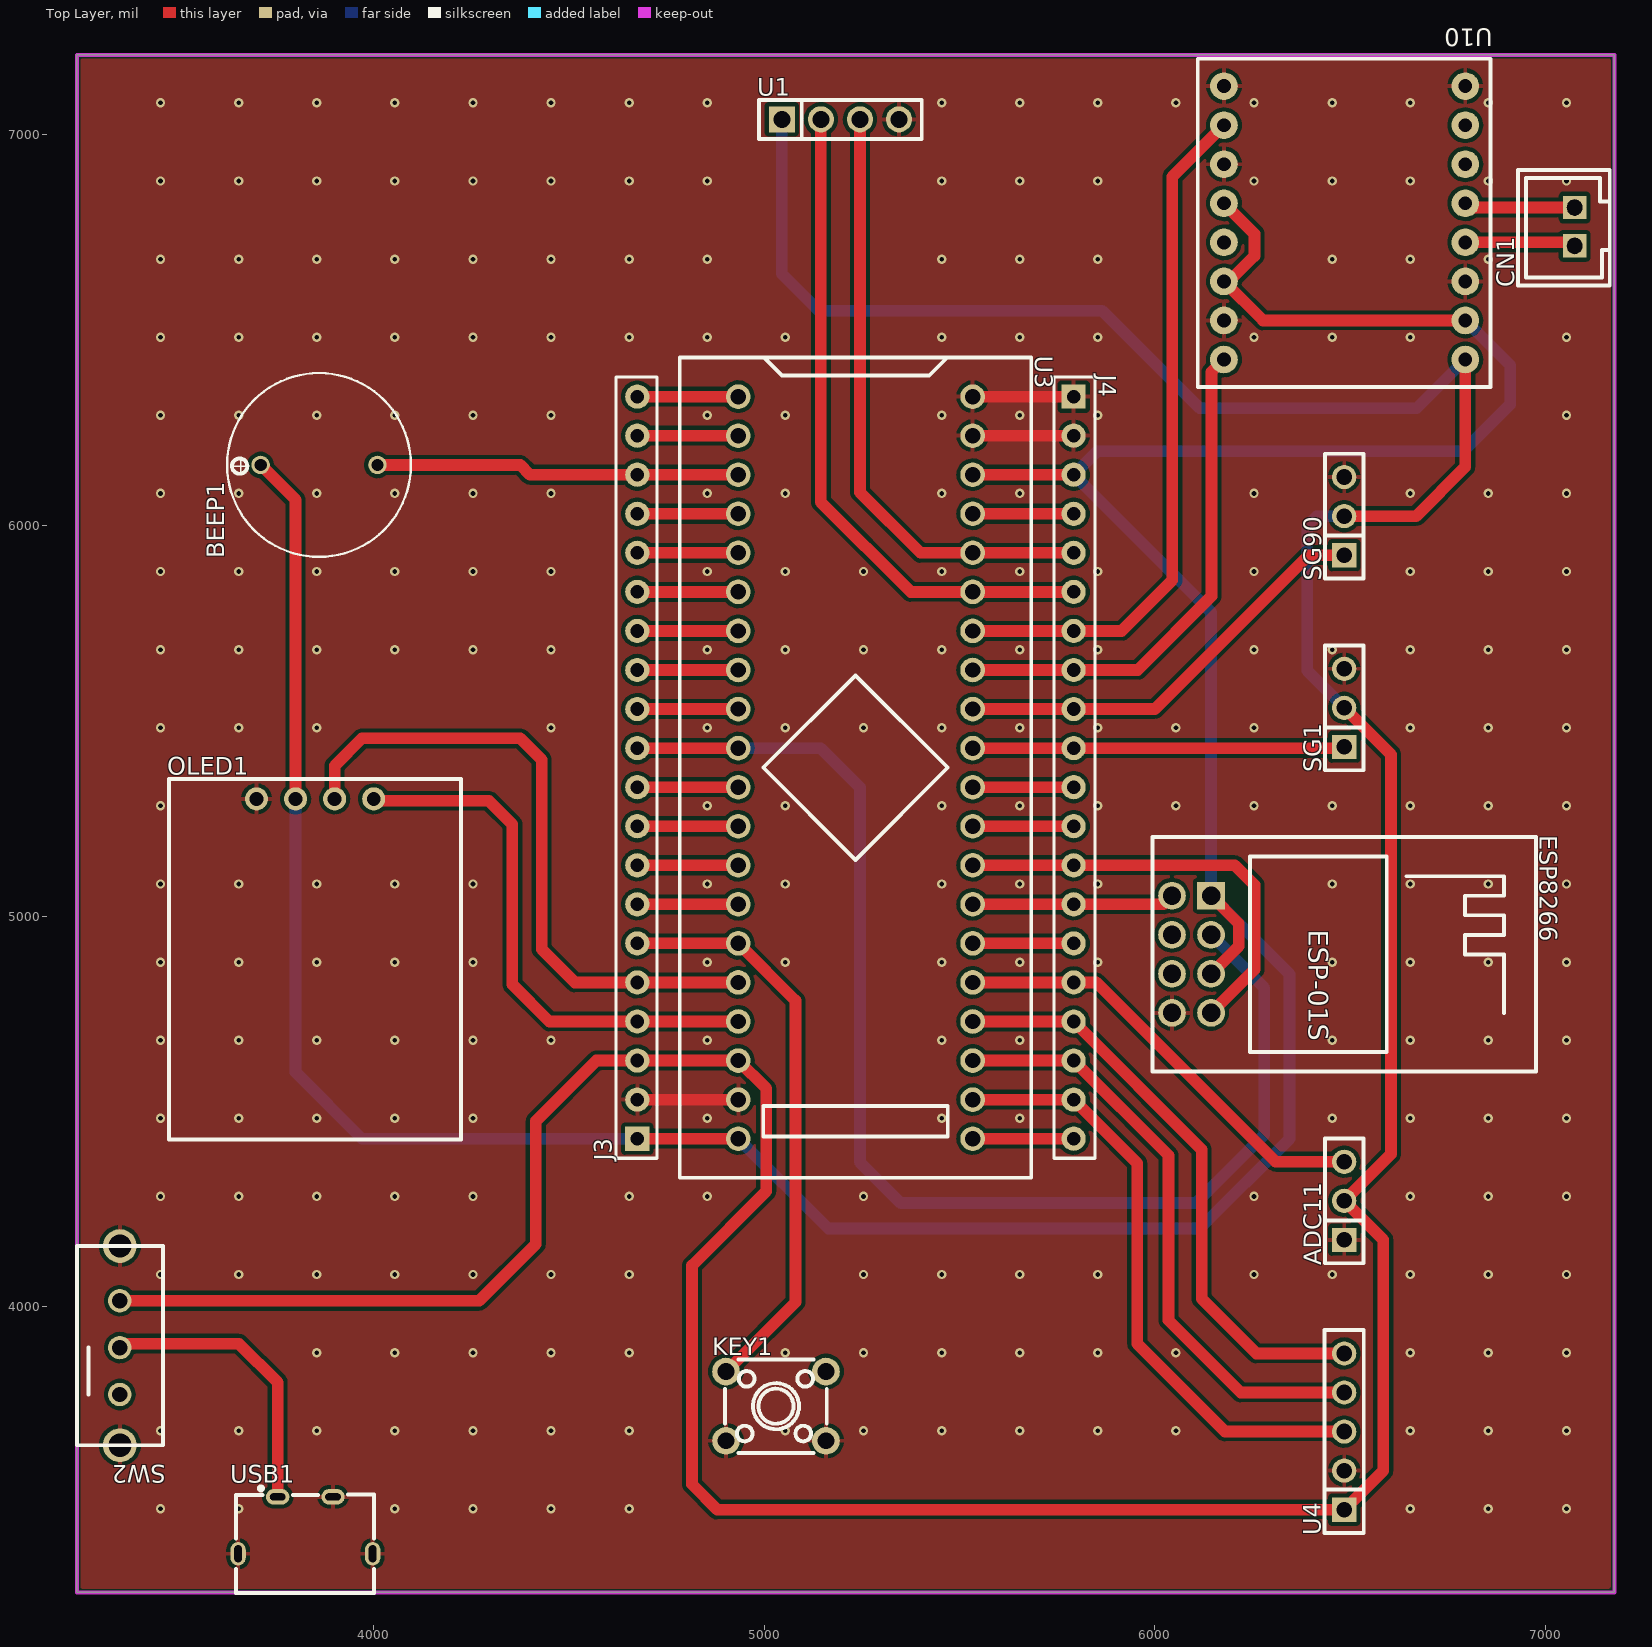
[diagram p0: Top Layer view]
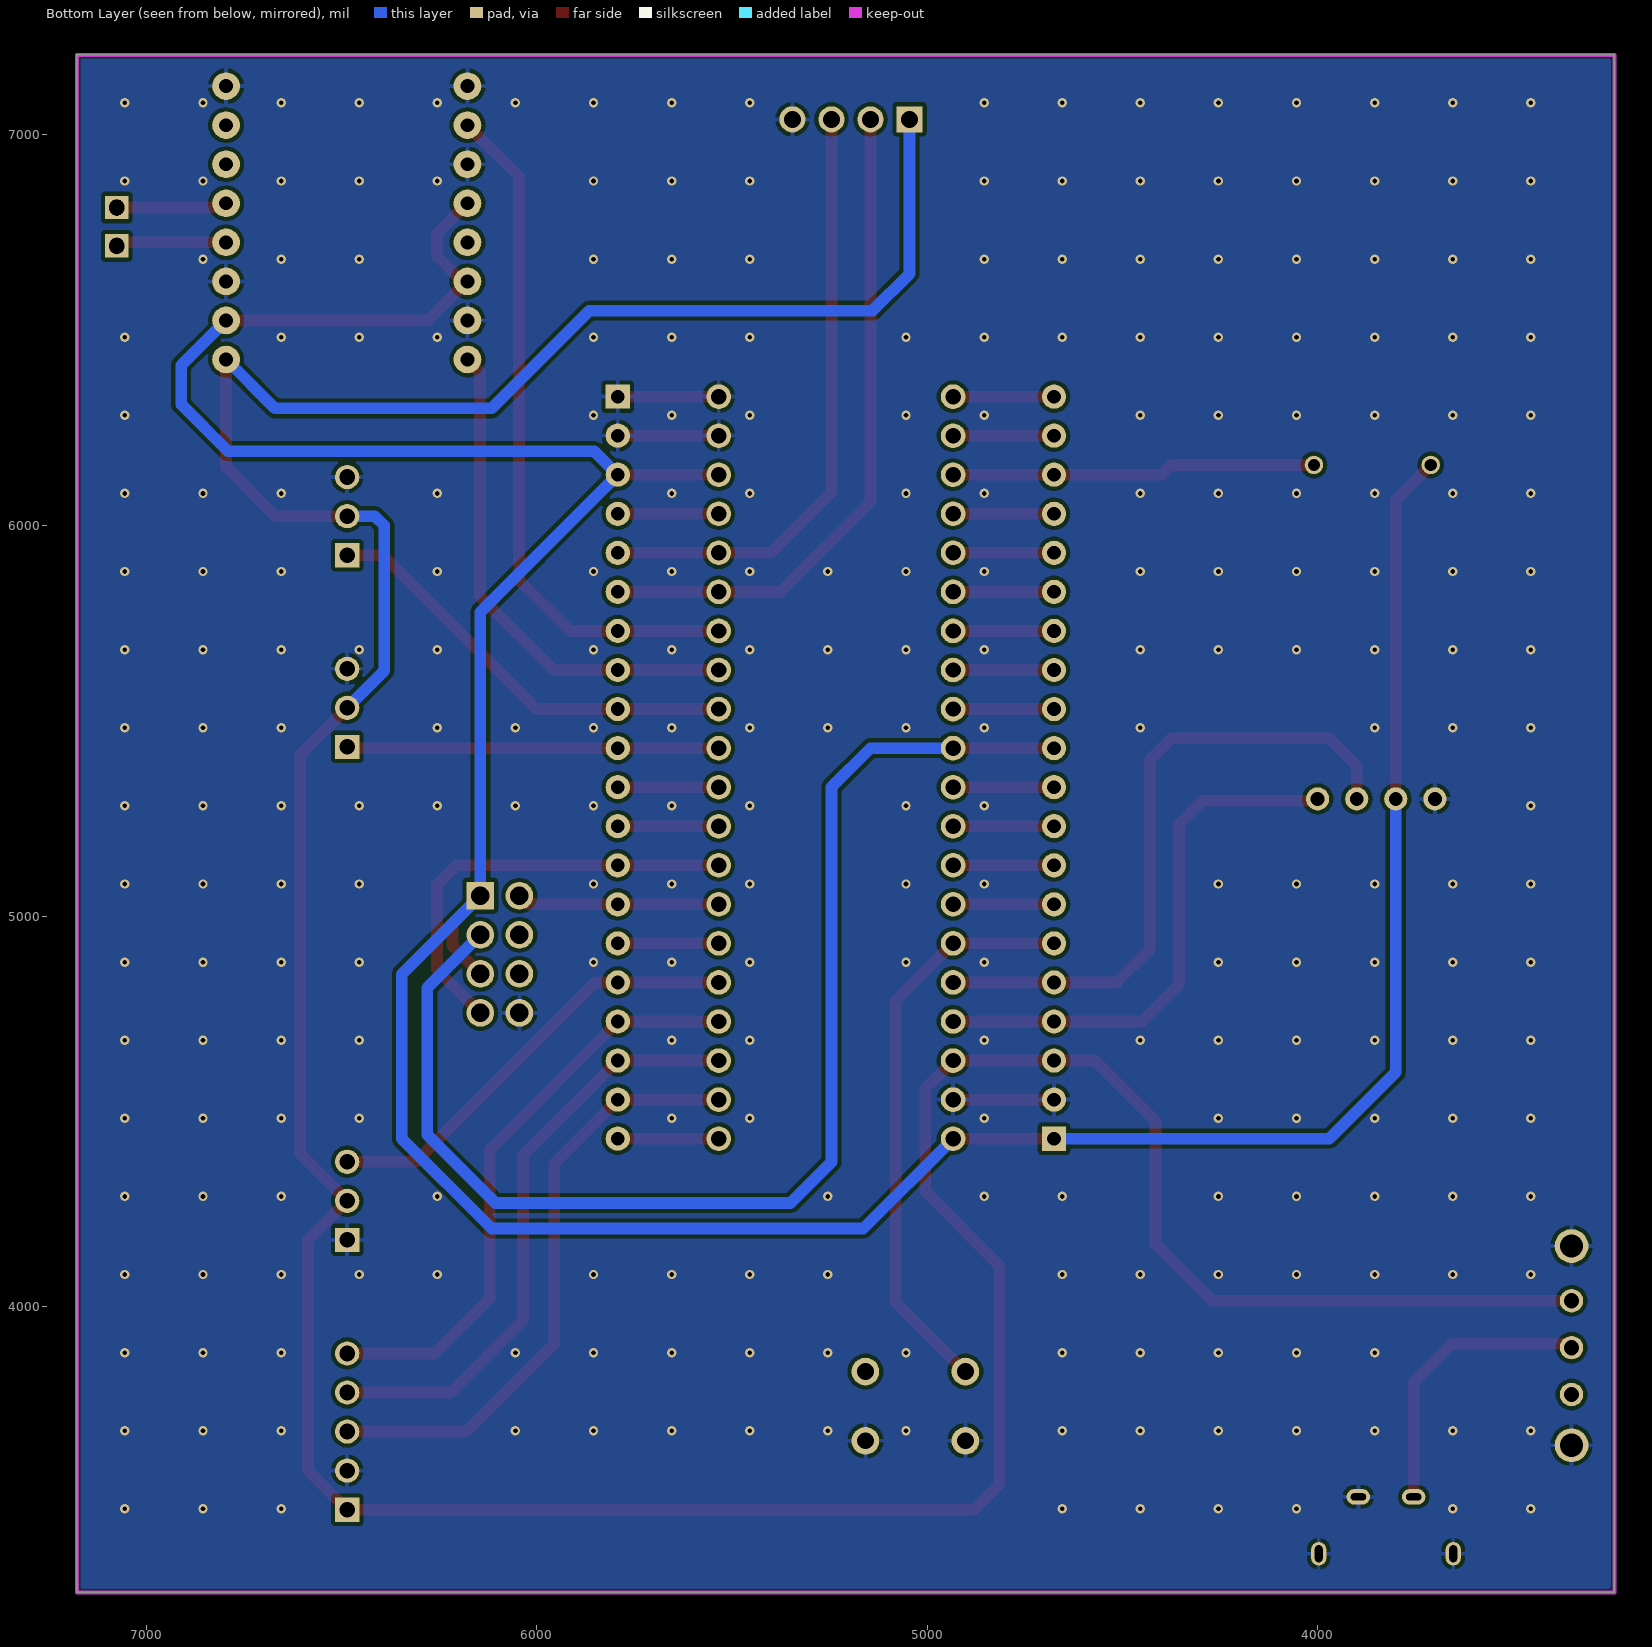
[diagram p1: Bottom Layer view, seen from below]
# Altium PCB MISC49936.pcbdoc
Units mil, origin at the board's own origin, x right, y up, seen from the top; angles counter-clockwise.
Board outline 3937.01 x 3937.01 mil, 2 copper layers (Top Layer, Bottom Layer), stack 62.206 mil thick; 16 components, 42 nets, 143 pads, 269 vias.

## Layer stack, top to bottom
Top Solder Mask Layer: solder mask 0.394, Dk 3.3
Top Layer: signal copper 1.379
Dielectric1: surface 59.449, FR4, Dk 4.5
Bottom Layer: signal copper 1.378
Bottom Solder Mask Layer: solder mask 0.394, Dk 3.3

## Board outline
3240,7205 3240,3267.99 7177.01,3267.99 7177.01,7205

## Design rules (kind name [scope] priority, off if disabled: settings)
BoardOutlineClearance copperThickness2oz_1 [All] p2 off: genericclearance=7.99 ignorepadtopadclearanceinfootprint=FALSE except(0: Arc-SplitContinuation Track-SplitContinuation SMDPad-SplitContinuation THPad-SplitContinuation Via-SplitContinuation Fill-SplitContinuation Region-SplitContinuation Poly-SplitContinuation Text-SplitContinuation Hole-SplitContinuation; 5.98: Arc-CutoutEdge SMDPad-CutoutEdge THPad-CutoutEdge Via-CutoutEdge Fill-CutoutEdge Region-CutoutEdge Text-CutoutEdge; 6.93: Hole-OutlineEdge Hole-CutoutEdge; 10: Poly-OutlineEdge Poly-CutoutEdge; 11.81: Arc-OutlineEdge Track-OutlineEdge SMDPad-OutlineEdge THPad-OutlineEdge Via-OutlineEdge Fill-OutlineEdge Region-OutlineEdge Text-OutlineEdge Track-CutoutEdge)
BoardOutlineClearance copperThickness1oz_1 [All] p4: genericclearance=4.02 ignorepadtopadclearanceinfootprint=FALSE except(0: Arc-SplitContinuation Track-SplitContinuation SMDPad-SplitContinuation THPad-SplitContinuation Via-SplitContinuation Fill-SplitContinuation Region-SplitContinuation Poly-SplitContinuation Text-SplitContinuation Hole-SplitContinuation; 6: SMDPad-CutoutEdge THPad-CutoutEdge Via-CutoutEdge Fill-CutoutEdge Region-CutoutEdge Text-CutoutEdge; 6.93: Hole-OutlineEdge Hole-CutoutEdge; 10: Poly-OutlineEdge Poly-CutoutEdge; 11.8: Arc-OutlineEdge Track-OutlineEdge SMDPad-OutlineEdge THPad-OutlineEdge Via-OutlineEdge Fill-OutlineEdge Region-OutlineEdge Text-OutlineEdge; 11.81: Arc-CutoutEdge Track-CutoutEdge)
Clearance copperThickness2oz [All] p1 off: gap=7.99 ignorepadtopadclearanceinfootprint=FALSE except(5.98: SMDPad-Track SMDPad-SMDPad THPad-Track SMDPad-THPad THPad-THPad Track-Via SMDPad-Via THPad-Via Via-Via Fill-Track Region-Track Fill-SMDPad Region-SMDPad Fill-THPad Region-THPad Fill-Via Region-Via Fill-Fill Fill-Region Region-Region Arc-Track Arc-SMDPad Arc-THPad Arc-Via Fill-Arc Region-Arc Arc-Arc Text-Track SMDPad-Text Text-THPad Text-Via Fill-Text Region-Text Arc-Text Text-Text; 6.93: Hole-Track Hole-SMDPad Hole-THPad Hole-Via Fill-Hole Region-Hole Hole-Arc Hole-Text; 10: Poly-Track Poly-SMDPad Poly-THPad Poly-Via Poly-Fill Poly-Region Poly-Poly Poly-Arc Poly-Text Poly-Hole)
Clearance copperThickness1oz [All] p3: gap=4.02 ignorepadtopadclearanceinfootprint=FALSE except(5.98: SMDPad-Track SMDPad-SMDPad THPad-Track SMDPad-THPad THPad-THPad Track-Via SMDPad-Via THPad-Via Via-Via Fill-Track Region-Track Fill-SMDPad Region-SMDPad Fill-THPad Region-THPad Fill-Via Region-Via Fill-Fill Fill-Region Region-Region; 6: Arc-Track Arc-SMDPad Arc-THPad Arc-Via Fill-Arc Region-Arc Arc-Arc Text-Track SMDPad-Text Text-THPad Text-Via Fill-Text Region-Text Arc-Text Text-Text; 6.93: Hole-Track Hole-SMDPad Hole-THPad Hole-Via Fill-Hole Region-Hole Hole-Arc Hole-Text; 10: Poly-Track Poly-SMDPad Poly-THPad Poly-Via Poly-Fill Poly-Region Poly-Poly Poly-Arc Poly-Text Poly-Hole)
DiffPairsRouting differentialPair [All] p1: maxlimit=6 minlimit=6 mostfreqgap=6 toplayer_minwidth=5 toplayer_prefwidth=10 toplayer_maxwidth=100 toplayer_mingap=6 toplayer_prefgap=6 toplayer_maxgap=6 bottomlayer_minwidth=5 bottomlayer_prefwidth=10 bottomlayer_maxwidth=100 bottomlayer_mingap=6 bottomlayer_prefgap=6 bottomlayer_maxgap=6 maxuncoupledlength=10
HoleToHoleClearance otherClearance [All] p1: gap=11.81 allowstackedmicrovias=TRUE
Length netLength [All] p1: minlimit=0 maxlimit=0
MatchedLengths netLengthTolerance [All] p1: tolerance=1000
PasteMaskExpansion pasteMaskExpansion [All] p1: expansion=0
PlaneConnect innerPlane [All] p1: planeconnectstyle=Relief reliefexpansion=20 reliefentries=4 reliefconductorwidth=10 reliefairgap=10
PolygonConnect copperRegion [(InNet('GND'))] p1: connectstyle=Relief reliefconductorwidth=10 reliefentries=4 polygonreliefangle="90 Angle" airgapwidth=10 via.connectstyle=Relief via.reliefconductorwidth=10 via.reliefentries=4 via.polygonreliefangle="90 Angle" via.airgapwidth=10
RoutingVias viaSize [All] p1: holewidth=12.01 width=24.02 viastyle="Through Hole" minholewidth=11.81 minwidth=19.68 maxholewidth=248.03 maxwidth=393.7
SolderMaskExpansion solderMaskExpansion [IsVia] p1: expansion=-1000 istentingtop=TRUE
SolderMaskExpansion solderMaskExpansion [All] p2: expansion=2 istentingtop=FALSE
Width copperThickness2oz_2 [All] p1 off: maxlimit=100 minlimit=8 preferedwidth=10
Width copperThickness1oz_2 [All] p2: maxlimit=100 minlimit=5 preferedwidth=10

## Components (designator, comment, footprint, x,y, rotation, side; value= is the part's Value field where it differs from the comment)
ADC11 "MQ135" HDR-TH_3P-P2.54-V-F 6485,4270.87 r90 top
BEEP1 "Buzzer" BUZ-TH_BD11.8-P7.60_XHXDZ-TMB12065 3860,6155 r90 top
CN1 "XH2.54-2PIN-straight pin" CONN-TH_XH2.54-2P 7075,6765 r90 top
ESP8266 "ESP-01S module" WIFIM-TH_ESP-01S 6094,4901.99 r270 top
J3 "HDR-M-2.54_1x20" HDR-M-2.54_1X20 4675,5380 r90 top
J4 "HDR-M-2.54_1x20" HDR-M-2.54_1X20 5792.09,5380 r270 top
KEY1 "K4-6×6_TH" KEY-TH_4P-L6.0-W6.0-P4.50-LS6.5 5030,3745 r0 top
OLED1 "0.96 OLED IIC COPY" OLED-TH_4P-L23.44-W19.0_ER-OLEDM0.66-1W-I2C 3850,5300 r0 top
SG1 "Servo" HDR-TH_3P-P2.54-V-F 6485,5533.11 r90 top
SG90 "Servo" HDR-TH_3P-P2.54-V-F 6485,6023.98 r90 top
SW2 "SK-12E12-G5" SW-TH_SK-12E12-G5 3350,3900 r180 top
U1 "HX711" HDR-TH_4P-P2.54-V-F 5195,7040 r0 top
U3 "STM32F103C8T6-Card" CONN-TH_L53.3-W22.9_STM32F103C8T6-CARD 5233.54,5380 r270 top
U4 "Clock DS1302" HDR-TH_5P-P2.54-V-F 6485,3680 r90 top
U10 "TB6612FNG" tb6612 6795,6425 r180 top
USB1 "KH-TYPE-C-2P" USB-SMD_KH-TYPE-C-2P 3825,3440 r0 top

## Footprints (in the part's own frame and the unit in brackets; to place one, negate y for a bottom-side part, rotate by r counter-clockwise, add the part's x,y. Pads: shape width x height; smd on the part's side, far side on the other; paste and mask are expansions set on the pad)
BUZ-TH_BD11.8-P7.60_XHXDZ-TMB12065 [mm]
  round 1.201 hole 0.801: 1(0,3.8) 2(0,-3.8)
  silkscreen extent -5.98,-5.98 5.98,5.98
CONN-TH_L53.3-W22.9_STM32F103C8T6-CARD [mm]
  round 1.6 hole 1: 1(-24.13,-7.62) 2(-21.59,-7.62) 3(-19.05,-7.62) 4(-16.51,-7.62) 5(-13.97,-7.62) 6(-11.43,-7.62) 7(-8.89,-7.62) 8(-6.35,-7.62) 9(-3.81,-7.62) 10(-1.27,-7.62) 11(1.27,-7.62) 12(3.81,-7.62) 13(6.35,-7.62) 14(8.89,-7.62) 15(11.43,-7.62) 16(13.97,-7.62) 17(16.51,-7.62) 18(19.05,-7.62) 19(21.59,-7.62) 20(24.13,-7.62) 21(24.13,7.62) 22(21.59,7.62) 23(19.05,7.62) 24(16.51,7.62) 25(13.97,7.62) 26(11.43,7.62) 27(8.89,7.62) 28(6.35,7.62) 29(3.81,7.62) 30(1.27,7.62) 31(-1.27,7.62) 32(-3.81,7.62) 33(-6.35,7.62) 34(-8.89,7.62) 35(-11.43,7.62) 36(-13.97,7.62) 37(-16.51,7.62) 38(-19.05,7.62) 39(-21.59,7.62) 40(-24.13,7.62)
  silkscreen extent -26.67,-11.43 26.67,11.43
CONN-TH_XH2.54-2P [mil]
  rect 60x60 hole 39.37 slot 41.34 at 0 deg paste+0 mask+1.97: 1(-49.22,0) 2(49.21,0)
  silkscreen extent -150,-90 145,145
HDR-M-2.54_1X20 [mil]
  rect 62x62 hole 35: 1(-950,0)
  round 62 hole 35: 2(-850,0) 3(-750,0) 4(-650,0) 5(-550,0) 6(-450,0) 7(-350,0) 8(-250,0) 9(-150,0) 10(-50,0) 11(50,0) 12(150,0) 13(250,0) 14(350,0) 15(450,0) 16(550,0) 17(650,0) 18(750,0) 19(850,0) 20(950,0)
  silkscreen extent -1000,-50 1000,55
HDR-TH_3P-P2.54-V-F [mil]
  rect 62x62 hole 40.16: 1(-100,0)
  round 62 hole 40.16: 2(0,0) 3(100,0)
  silkscreen extent -160,-49 160,49
HDR-TH_4P-P2.54-V-F [mm]
  rect 1.7x1.7 hole 1.1: 1(-3.81,0)
  round 1.7 hole 1.1: 2(-1.27,0) 3(1.27,0) 4(3.81,0)
  silkscreen extent -5.29,-1.27 5.29,1.27
HDR-TH_5P-P2.54-V-F [mil]
  rect 62x62 hole 40.16: 1(-200,0)
  round 62 hole 40.16: 2(-100,0) 3(0,0) 4(100,0) 5(200,0)
  silkscreen extent -260,-50 260,50
KEY-TH_4P-L6.0-W6.0-P4.50-LS6.5 [mm]
  round 1.8 hole 1.1: 1(-3.251,-2.25) 2(3.251,-2.25) 3(3.251,2.25) 4(-3.251,2.25)
  silkscreen extent -3.3,-3.05 3.3,3.05
OLED-TH_4P-L23.44-W19.0_ER-OLEDM0.66-1W-I2C [mm]
  round 1.5 hole 0.9 paste+0 mask+0.05: 1(-3.81,0) 2(-1.27,0) 3(1.27,0) 4(3.81,0)
  silkscreen extent -9.5,-22.15 9.5,1.3
SW-TH_SK-12E12-G5 [mil]
  round 60 hole 39.37: 1(0,125) 2(0,5) 3(0,-115)
  round 86.61 hole 59.06: 4(0,-255) 5(0,255)
  silkscreen extent -110,-255 110,255
tb6612 [mm]
  round 1.8 hole 0.9: 1(0,0) 2(0,-2.54) 3(0,-5.08) 4(0,-7.62) 5(0,-10.16) 6(0,-12.7) 7(0,-15.24) 8(0,-17.78) 9(15.697,-17.78) 10(15.697,-15.24) 11(15.697,-12.7) 12(15.697,-10.16) 13(15.697,-7.62) 14(15.697,-5.08) 15(15.697,-2.54) 16(15.697,0)
  silkscreen extent -1.65,-19.56 17.4,1.78
USB-SMD_KH-TYPE-C-2P [mm]
  oval 1.524x1 hole 0.45 slot 1 at 0 deg paste+0 mask+0.05: 1(-1.8,1.85) 2(1.8,1.85)
  oval 1x1.524 hole 0.5 slot 1.1 at 90 deg paste+0 mask+0.05: 3(4.375,-1.85) 4(-4.375,-1.85)
  silkscreen extent -4.5,-4.41 4.46,2.53
WIFIM-TH_ESP-01S [mm]
  rect 1.8x1.8 hole 1.2: 1(-3.81,1.27)
  round 1.8 hole 1.2: 2(-1.27,1.27) 3(1.27,1.27) 4(3.81,1.27) 5(3.81,-1.27) 6(1.27,-1.27) 7(-1.27,-1.27) 8(-3.81,-1.27)
  silkscreen extent -7.62,-2.54 7.62,22.4

## Via types
v1: diameter 24.02, hole 12, Top Layer to Bottom Layer, 269 vias

## Nets (pads, with @x,y where several pads share a name; then routed paths per layer and width w, separated by ;. In a path a pad name is that pad's centre, name@x,y a point inside that pad or via, vN(x,y) a via of type N, cw(c..) or ccw(c..) an arc to the next point about the centre after c; other vN are vias at no path point)
$2N25: SW2.2 USB1.1 | length 738.2
  Top Layer w30: SW2.2@3350,3905 3655,3905 3754.13,3805.87 USB1.1
$2N63: J4.12 U3.29 | length 271.5
  Top Layer w30: U3.29 J4.12@5805,5230
$2N68: J4.4 U3.37 | length 271.5
  Top Layer w30: U3.37 J4.4@5805,6030
$2N71: J4.11 U3.30 | length 271.5
  Top Layer w30: U3.30 J4.11@5805,5330
$2N78: J3.10 U3.11 | length 258.5
  Top Layer w30: J3.10 U3.11
$2N81: J4.20 U3.21 | length 271.5
  Top Layer w30: U3.21 J4.20@5805,4430
+5V: ADC11.2 J3.3 SG1.2 SG90.2 SW2.3 U1.1 U3.18 U4.1 U10.1 | length 10736.4
  Top Layer w30: SW2.3 4270,4015 4415,4160 4415,4475 4570,4630 J3.3 U3.18 5005,4558.54 5005,4295 4815,4105 4815,3545 4880,3480 U4.1 6585,3580 6585,4170.87 ADC11.2 6605,4390.87 6605,5413.11 SG1.2 ; SG90.2 6668.98,6023.98 6795,6150 U10.1
  Bottom Layer w30: U1.1 5045,6645 5140,6550 5865,6550 6115,6300 6670,6300 U10.1 ; SG1.2 6390,5628.11 6390,6000 6413.98,6023.98 SG90.2
ADC1_0: ADC11.3 J4.16 U3.25 | length 1141.6
  Top Layer w30: U3.25 J4.16 5850,4830 6309.13,4370.87 ADC11.3
ADC1_1: J4.15 U3.26 | length 271.5
  Top Layer w30: U3.26 J4.15@5805,4930
AO1: CN1.1 U10.4 | length 283.8
  Top Layer w30: U10.4 7065.78,6725 CN1.1
AO2: CN1.2 U10.5 | length 284.5
  Top Layer w30: U10.5 6805.78,6814.22 CN1.2
BEEP: BEEP1.2 J3.18 U3.3 | length 934.3
  Top Layer w30: BEEP1.2 4375,6155 4400,6130 J3.18 U3.3
BO1: U10.7
BO2: U10.6
DATA_DS: J4.18 U3.23 U4.4 | length 1550.8
  Top Layer w30: U3.23 J4.18 6035,4387.08 6035,3965 6220,3780 U4.4
DATA_HX: J4.5 U1.3 U3.36 | length 1579.2
  Top Layer w30: U1.3 5245,6085 5400,5930 U3.36 J4.5@5805,5930
DO: J3.12 U3.9 | length 258.5
  Top Layer w30: J3.12 U3.9
DUOJI: J4.9 SG90.1 U3.32 | length 1114.6
  Top Layer w30: U3.32 J4.9 6000,5530 6393.98,5923.98 SG90.1
ECHO: J4.10 SG1.1 U3.31 | length 952.7
  Top Layer w30: U3.31 J4.10 6481.89,5430 SG1.1
GND: ADC11.1 ESP8266.5 J3.2 J4.1 J4.2 KEY1.1 KEY1.2 OLED1.1 SG1.3 SG90.3 SW2.4 SW2.5 U1.4 U3.19 U3.39 U3.40 U4.2 U10.3 U10.8 U10.9 U10.11 U10.15 USB1.2 USB1.3 USB1.4 | length 801.5
  Top Layer w30: J3.2 U3.19 ; U3.39 J4.2@5805,6230 ; U3.40 J4.1@5805,6330
  other v1: 3454.1,3482.09 3654.1,3482.09 4054.1,3482.09 4254.1,3482.09 4454.1,3482.09 4654.1,3482.09 6654.1,3482.09 6854.1,3482.09 7054.1,3482.09 3454.1,3682.09 3654.1,3682.09 3854.1,3682.09 4054.1,3682.09 4254.1,3682.09 4454.1,3682.09 4654.1,3682.09 5054.1,3682.09 5254.1,3682.09 5454.1,3682.09 5654.1,3682.09 5854.1,3682.09 6054.1,3682.09 6654.1,3682.09 6854.1,3682.09 7054.1,3682.09 3854.1,3882.09 4054.1,3882.09 4254.1,3882.09 4454.1,3882.09 4654.1,3882.09 5054.1,3882.09 5254.1,3882.09 5454.1,3882.09 5654.1,3882.09 5854.1,3882.09 6054.1,3882.09 6654.1,3882.09 6854.1,3882.09 7054.1,3882.09 3454.1,4082.09 3654.1,4082.09 3854.1,4082.09 4054.1,4082.09 4254.1,4082.09 4454.1,4082.09 4654.1,4082.09 5254.1,4082.09 5454.1,4082.09 5654.1,4082.09 5854.1,4082.09 6254.1,4082.09 6454.1,4082.09 6654.1,4082.09 6854.1,4082.09 7054.1,4082.09 3454.1,4282.09 3654.1,4282.09 3854.1,4282.09 4054.1,4282.09 4254.1,4282.09 4654.1,4282.09 4854.1,4282.09 5254.1,4282.09 6254.1,4282.09 6654.1,4282.09 6854.1,4282.09 7054.1,4282.09 3454.1,4482.09 3654.1,4482.09 3854.1,4482.09 4054.1,4482.09 4254.1,4482.09 4854.1,4482.09 5454.1,4482.09 5654.1,4482.09 6454.1,4482.09 6654.1,4482.09 6854.1,4482.09 7054.1,4482.09 3454.1,4682.09 3654.1,4682.09 3854.1,4682.09 4054.1,4682.09 4254.1,4682.09 4454.1,4682.09 4854.1,4682.09 5454.1,4682.09 5654.1,4682.09 6454.1,4682.09 6654.1,4682.09 6854.1,4682.09 7054.1,4682.09 3454.1,4882.09 3654.1,4882.09 3854.1,4882.09 4054.1,4882.09 4254.1,4882.09 4854.1,4882.09 5054.1,4882.09 5454.1,4882.09 5654.1,4882.09 5854.1,4882.09 6454.1,4882.09 6654.1,4882.09 6854.1,4882.09 7054.1,4882.09 3454.1,5082.09 3654.1,5082.09 3854.1,5082.09 4054.1,5082.09 4254.1,5082.09 4854.1,5082.09 5054.1,5082.09 5454.1,5082.09 5654.1,5082.09 5854.1,5082.09 6454.1,5082.09 6654.1,5082.09 6854.1,5082.09 7054.1,5082.09 3454.1,5282.09 4854.1,5282.09 5054.1,5282.09 5454.1,5282.09 5654.1,5282.09 5854.1,5282.09 6054.1,5282.09 6254.1,5282.09 6454.1,5282.09 6654.1,5282.09 6854.1,5282.09 7054.1,5282.09 3454.1,5482.09 3654.1,5482.09 3854.1,5482.09 4454.1,5482.09 4854.1,5482.09 5054.1,5482.09 5254.1,5482.09 5454.1,5482.09 5654.1,5482.09 5854.1,5482.09 6054.1,5482.09 6254.1,5482.09 6654.1,5482.09 6854.1,5482.09 7054.1,5482.09 3454.1,5682.09 3654.1,5682.09 3854.1,5682.09 4054.1,5682.09 4254.1,5682.09 4454.1,5682.09 4854.1,5682.09 5054.1,5682.09 5254.1,5682.09 5454.1,5682.09 5654.1,5682.09 5854.1,5682.09 6254.1,5682.09 6454.1,5682.09 6654.1,5682.09 6854.1,5682.09 7054.1,5682.09 3454.1,5882.09 3654.1,5882.09 3854.1,5882.09 4054.1,5882.09 4254.1,5882.09 4454.1,5882.09 4854.1,5882.09 5054.1,5882.09 5254.1,5882.09 5454.1,5882.09 5654.1,5882.09 5854.1,5882.09 6254.1,5882.09 6654.1,5882.09 6854.1,5882.09 7054.1,5882.09 3454.1,6082.09 3654.1,6082.09 3854.1,6082.09 4054.1,6082.09 4254.1,6082.09 4454.1,6082.09 4854.1,6082.09 5054.1,6082.09 5454.1,6082.09 5654.1,6082.09 6254.1,6082.09 6654.1,6082.09 6854.1,6082.09 7054.1,6082.09 3454.1,6282.09 3654.1,6282.09 3854.1,6282.09 4054.1,6282.09 4254.1,6282.09 4454.1,6282.09 4854.1,6282.09 5054.1,6282.09 5454.1,6282.09 5654.1,6282.09 5854.1,6282.09 7054.1,6282.09 3454.1,6482.09 3654.1,6482.09 3854.1,6482.09 4054.1,6482.09 4254.1,6482.09 4454.1,6482.09 4654.1,6482.09 4854.1,6482.09 5054.1,6482.09 5454.1,6482.09 5654.1,6482.09 5854.1,6482.09 6254.1,6482.09 6454.1,6482.09 6654.1,6482.09 7054.1,6482.09 3454.1,6682.09 3654.1,6682.09 3854.1,6682.09 4054.1,6682.09 4254.1,6682.09 4454.1,6682.09 4654.1,6682.09 4854.1,6682.09 5454.1,6682.09 5654.1,6682.09 5854.1,6682.09 6454.1,6682.09 6654.1,6682.09 6854.1,6682.09 3454.1,6882.09 3654.1,6882.09 3854.1,6882.09 4054.1,6882.09 4254.1,6882.09 4454.1,6882.09 4654.1,6882.09 4854.1,6882.09 5454.1,6882.09 5654.1,6882.09 5854.1,6882.09 6254.1,6882.09 6454.1,6882.09 6654.1,6882.09 6854.1,6882.09 7054.1,6882.09 3454.1,7082.09 3654.1,7082.09 3854.1,7082.09 4054.1,7082.09 4254.1,7082.09 4454.1,7082.09 4654.1,7082.09 4854.1,7082.09 5454.1,7082.09 5654.1,7082.09 5854.1,7082.09 6054.1,7082.09 6254.1,7082.09 6454.1,7082.09 6654.1,7082.09 6854.1,7082.09 7054.1,7082.09
JDQ: J3.19 U3.2 | length 258.5
  Top Layer w30: J3.19 U3.2
KEY1: J3.6 KEY1.4 U3.15 | length 1489.3
  Top Layer w30: J3.6 U3.15 5080,4783.54 5080,4011.6 KEY1.4
KEY2: J3.7 U3.14 | length 258.5
  Top Layer w30: J3.7 U3.14
KEY3: J3.9 U3.12 | length 258.5
  Top Layer w30: J3.9 U3.12
LED: J3.20 U3.1 | length 258.5
  Top Layer w30: J3.20 U3.1
LED2: J3.16 U3.5 | length 258.5
  Top Layer w30: J3.16 U3.5
PWMA: J4.8 U3.33 U10.16 | length 1309.2
  Top Layer w30: U3.33 J4.8 5956.42,5630 6145,5818.58 6145,6393 U10.16
PWMB: J4.7 U3.34 U10.10 | length 1785
  Top Layer w30: U3.34 J4.7 5915,5730 6045,5860 6045,6893 U10.10
RST_DS: J4.17 U3.24 U4.5 | length 1527.4
  Top Layer w30: U3.24 J4.17 6120,4402.08 6120,4020 6260,3880 U4.5
RST_ESP: ESP8266.2 J3.11 U3.10 | length 3290.7
  Top Layer w30: J3.11 U3.10
  Bottom Layer w30: U3.10 5145,5430 5245,5330 5245,4370 5350,4265 6105,4265 6280,4440 6280,4815.99 ESP8266.2
RX_6288: J3.15 U3.6 | length 258.5
  Top Layer w30: J3.15 U3.6
RX_ESP: ESP8266.8 J4.14 U3.27 | length 519.6
  Top Layer w30: U3.27 J4.14 6022.01,5030 ESP8266.8
SCK_HX: J4.6 U1.2 U3.35 | length 1735.3
  Top Layer w30: U1.2 5145,6060 5375,5830 U3.35 J4.6@5805,5830
SCL: J3.5 OLED1.3 U3.16 | length 1690.5
  Top Layer w30: OLED1.3 3900,5385 3970,5455 4375,5455 4430,5400 4430,4915 4515,4830 J3.5 U3.16
SCLK_DS: J4.19 U3.22 U4.3 | length 1574.2
  Top Layer w30: U3.22 J4.19 5955,4367.08 5955,3905 6180,3680 U4.3
SDA: J3.4 OLED1.4 U3.17 | length 1409.8
  Top Layer w30: OLED1.4 4005,5295 4295,5295 4355,5235 4355,4825 4450,4730 J3.4 U3.17
SR501: J3.13 U3.8 | length 258.5
  Top Layer w30: J3.13 U3.8
TEMP: J3.8 U3.13 | length 258.5
  Top Layer w30: J3.8 U3.13
TRIG: J3.17 U3.4 | length 258.5
  Top Layer w30: J3.17 U3.4
TX_6288: J3.14 U3.7 | length 258.5
  Top Layer w30: J3.14 U3.7
TX_ESP: ESP8266.4 J4.13 U3.28 | length 1116.2
  Top Layer w30: U3.28 J4.13 6205,5130 6255,5080 6255,4862.99 ESP8266.4
VCC: BEEP1.1 ESP8266.1 ESP8266.3 J3.1 J4.3 OLED1.2 U3.20 U3.38 U10.2 U10.12 U10.13 U10.14 | length 9244.1
  Top Layer w30: BEEP1.1 3800,6065.39 OLED1.2 ; J3.1 U3.20 ; U3.38 J4.3@5805,6130 ; ESP8266.3 6215,4922.99 6215,4980.99 ESP8266.1 ; U10.12 6255,6747 6255,6690 6190,6625 U10.14 6277,6525 U10.2
  Bottom Layer w30: OLED1.2 3800,4600 3970,4430 J3.1 ; U3.20 5163.54,4200 6115,4200 6345,4430 6345,4850.99 ESP8266.1 6144,5778.08 J4.3 5852.09,6190 6790,6190 6910,6310 6910,6410 U10.2
pads on no net: ESP8266.6 ESP8266.7 KEY1.3 SW2.1

## Polygon pours and split planes (outlines as drawn)
GND on Top Layer (solid, remove dead copper, pour order 0): 3000,7440 3000,3095 7525,3095 7525,7440
GND on Bottom Layer (solid, remove dead copper, pour order 2): 3155,7385 3155,3000 7495,3000 7495,7385

## Keep-outs
Board Outline Layer:
  the board outline again, w10